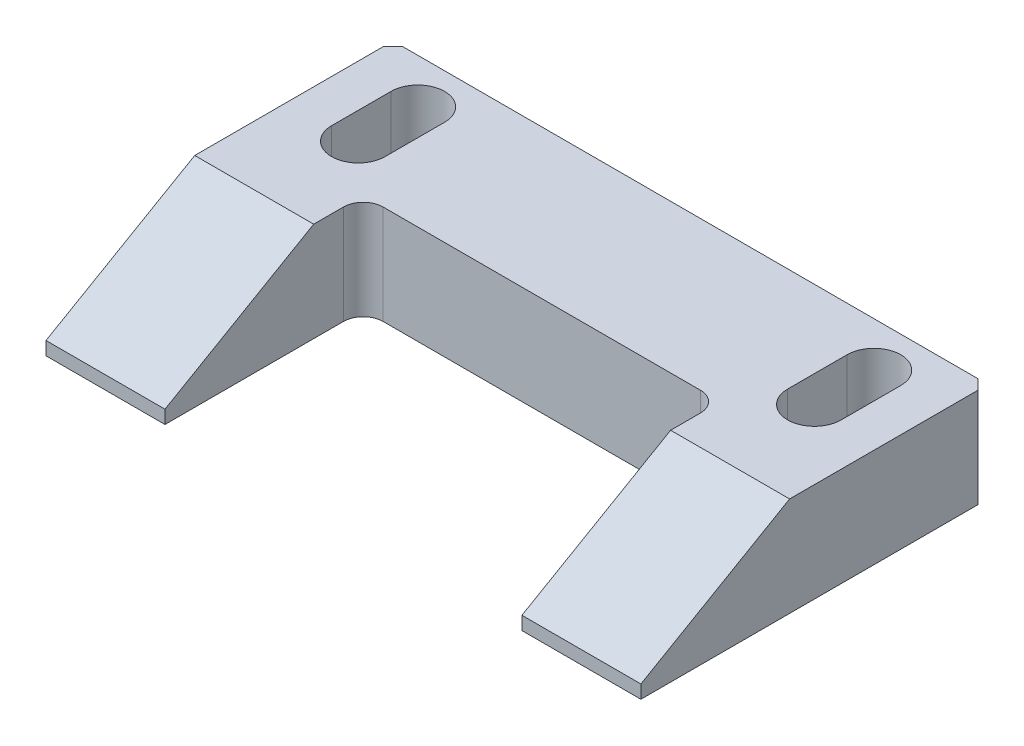
from build123d import *

# Parameters (mm, degrees)
SKETCH1_W           = 60
SKETCH1_H           = 35
BOSS_EXTRUDE1_DEPTH = 10
CHAMFER1_SIZE       = 15
CHAMFER1_SIZE2      = 8.660254038
SKETCH2_W           = 36
SKETCH2_H           = 20
CUT_EXTRUDE1_DEPTH  = 37.142080737
FILLET1_R           = 2
CUT_EXTRUDE2_DEPTH  = 37.142080737
CHAMFER2_SIZE       = 1


with BuildPart() as part:
    # Sketch1 → Boss-Extrude1 (new body)
    with BuildSketch(Plane(origin=(0, 0, 0), x_dir=(1, 0, 0), z_dir=(0, 1, 0))):
        Rectangle(SKETCH1_W, SKETCH1_H)
    extrude(amount=BOSS_EXTRUDE1_DEPTH)

    # Chamfer1
    chamfer1_edges = [part.edges().sort_by_distance(p)[0] for p in [
        (0, 10, 17.5),
    ]]
    chamfer1_side = [part.faces().sort_by_distance(p)[0] for p in [
        (0, 10, 0),
    ]]
    chamfer(chamfer1_edges, length=CHAMFER1_SIZE, length2=CHAMFER1_SIZE2, reference=chamfer1_side[0])

    # Sketch2 → Cut-Extrude1 (cut, through all)
    with BuildSketch(Plane(origin=(0, 10, 0), x_dir=(1, 0, 0), z_dir=(0, 1, 0))):
        with Locations((0, -7.5)):
            Rectangle(SKETCH2_W, SKETCH2_H)
    extrude(amount=-CUT_EXTRUDE1_DEPTH, mode=Mode.SUBTRACT)

    # Fillet1
    fillet1_edges = [part.edges().sort_by_distance(p)[0] for p in [
        (-18, 5, -2.5),
        (18, 5, -2.5),
    ]]
    fillet(fillet1_edges, radius=FILLET1_R)

    # Sketch3 → Cut-Extrude2 (cut, through all)
    with BuildSketch(Plane(origin=(0, 10, 0), x_dir=(1, 0, 0), z_dir=(0, 1, 0))):
        with BuildLine():
            Line((-20.3, 13), (-20.3, 7))
            ThreePointArc((-20.3, 7), (-23, 4.3), (-25.7, 7))
            Line((-25.7, 7), (-25.7, 13))
            ThreePointArc((-25.7, 13), (-23, 15.7), (-20.3, 13))
        make_face()
    cut_extrude2 = extrude(amount=-CUT_EXTRUDE2_DEPTH, mode=Mode.SUBTRACT)

    # Mirror1: Cut-Extrude2 across plane
    add(cut_extrude2.mirror(Plane(origin=(0, 0, 0), x_dir=(0, 0, 1), z_dir=(1, 0, 0))), mode=Mode.SUBTRACT)

    # Chamfer2
    chamfer2_edges = [part.edges().sort_by_distance(p)[0] for p in [
        (-30, 5, -17.5),
        (30, 5, -17.5),
    ]]
    chamfer(chamfer2_edges, length=CHAMFER2_SIZE)


solid = part.part
